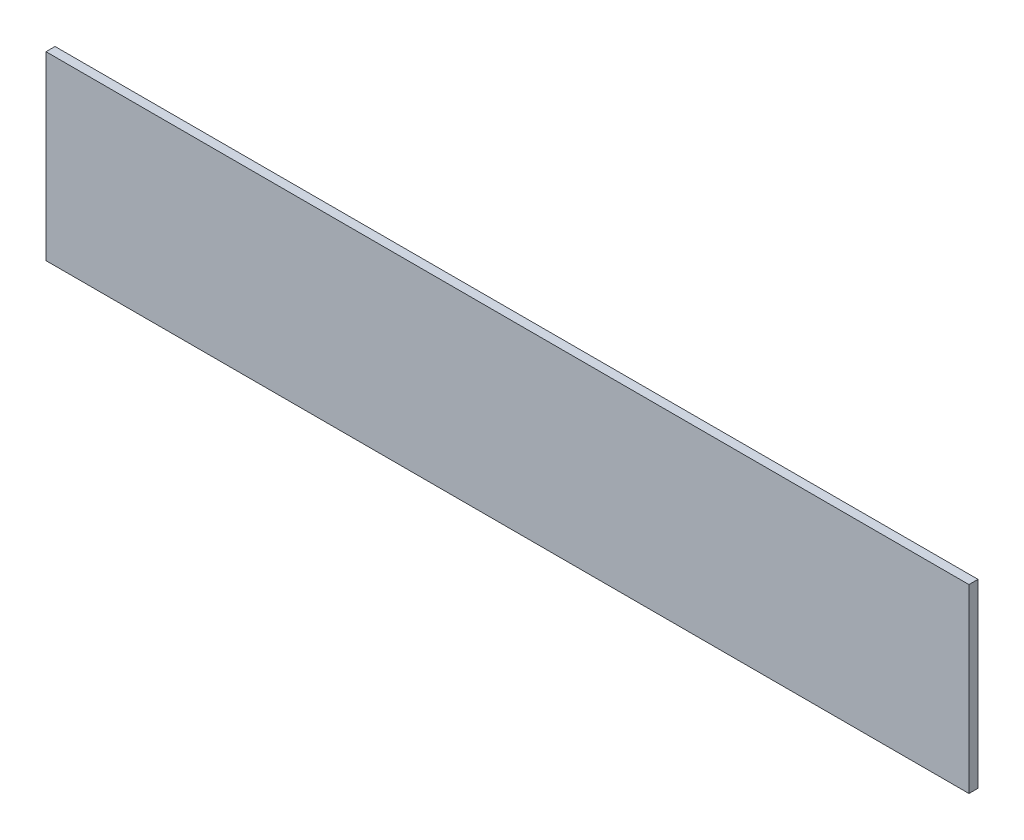
SolidWorks part; units mm, degrees
ref_plane "Front Plane" through (0, 0, 0) normal (0, 0, 1) x (1, 0, 0)
ref_plane "Top Plane" through (0, 0, 0) normal (0, 1, 0) x (1, 0, 0)
ref_plane "Right Plane" through (0, 0, 0) normal (1, 0, 0) x (0, 0, -1)
other "Configuration Table"
sketch "Sketch1" plane through (0, 0, 0) normal (0, 0, 1) x (1, 0, 0)
  line L1 (0, 0) -> (510, 0)
  line L2 (0, 0) -> (0, 100)
  line L3 (0, 100) -> (510, 100)
  line L4 (510, 0) -> (510, 100)
  dimension "D1" = 510
  dimension "D2" = 100
extrude "Boss-Extrude1" add sketch "Sketch1" along normal blind 5
